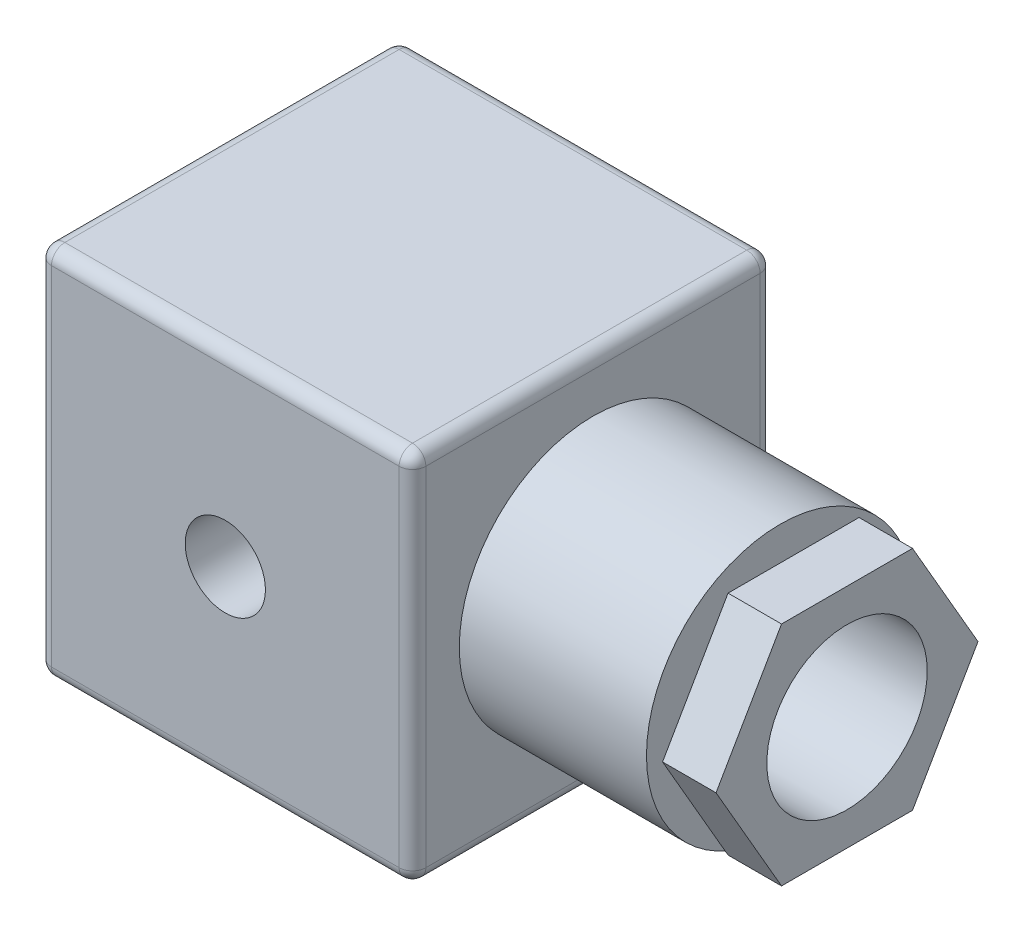
SolidWorks part; units mm, degrees
ref_plane "Front Plane" through (0, 0, 0) normal (0, 0, 1) x (1, 0, 0)
ref_plane "Top Plane" through (0, 0, 0) normal (0, 1, 0) x (1, 0, 0)
ref_plane "Right Plane" through (0, 0, 0) normal (1, 0, 0) x (0, 0, -1)
sketch "Sketch1" plane through (0, 0, 0) normal (0, 0, 1) x (1, 0, 0)
  line L0 (18.5, 7.0716) -> (18.5, 6.292) construction
  line L1 (18.5, 6.292) -> (18.7639, 6.292) construction
  line L2 (18.7639, 6.292) -> (18.7639, 6.6818) construction
  line L3 (18.7639, 6.6818) -> (21.2361, 6.6818) construction
  line L4 (21.2361, 6.6818) -> (21.2361, 6.292) construction
  line L5 (21.2361, 6.292) -> (21.5, 6.292) construction
  line L6 (21.5, 6.292) -> (21.5, 7.0716) construction
  line L7 (21.5, 7.0716) -> (18.5, 7.0716) construction
  line L8 (11.1066, -1.5169) -> (11.1066, 1.5169) construction
  line L9 (11.1066, 1.5169) -> (10.5248, 1.5169) construction
  line L10 (10.5248, 1.5169) -> (10.5248, -1.5169) construction
  line L11 (10.5248, -1.5169) -> (11.1066, -1.5169) construction
  line L12 (18.5, -6.292) -> (18.5, -7.0716) construction
  line L13 (18.5, -7.0716) -> (21.5, -7.0716) construction
  line L14 (21.5, -7.0716) -> (21.5, -6.292) construction
  line L15 (21.5, -6.292) -> (21.2361, -6.292) construction
  line L16 (21.2361, -6.292) -> (21.2361, -6.6818) construction
  line L17 (21.2361, -6.6818) -> (18.7639, -6.6818) construction
  line L18 (18.7639, -6.6818) -> (18.7639, -6.292) construction
  line L19 (18.7639, -6.292) -> (18.5, -6.292) construction
  line L20 (18.5, 7.0716) -> (18.5, 6.292)
  line L21 (18.5, 6.292) -> (18.7639, 6.292)
  line L22 (18.7639, 6.292) -> (18.7639, 6.6818)
  line L23 (18.7639, 6.6818) -> (21.2361, 6.6818)
  line L24 (21.2361, 6.6818) -> (21.2361, 6.292)
  line L25 (21.2361, 6.292) -> (21.5, 6.292)
  line L26 (21.5, 6.292) -> (21.5, 7.0716)
  line L27 (21.5, 7.0716) -> (18.5, 7.0716)
  line L28 (11.1066, -1.5169) -> (11.1066, 1.5169)
  line L29 (11.1066, 1.5169) -> (10.5248, 1.5169)
  line L30 (10.5248, 1.5169) -> (10.5248, -1.5169)
  line L31 (10.5248, -1.5169) -> (11.1066, -1.5169)
  line L32 (18.5, -6.292) -> (18.5, -7.0716)
  line L33 (18.5, -7.0716) -> (21.5, -7.0716)
  line L34 (21.5, -7.0716) -> (21.5, -6.292)
  line L35 (21.5, -6.292) -> (21.2361, -6.292)
  line L36 (21.2361, -6.292) -> (21.2361, -6.6818)
  line L37 (21.2361, -6.6818) -> (18.7639, -6.6818)
  line L38 (18.7639, -6.6818) -> (18.7639, -6.292)
  line L39 (18.7639, -6.292) -> (18.5, -6.292)
  line L40 (17, -6) -> (17, 6) construction
  line L41 (3, 14) -> (31, 14)
  line L42 (3, 14) -> (3, -14)
  line L43 (3, -14) -> (31, -14)
  line L44 (31, 14) -> (31, -14)
  line L45 (3, 14) -> (31, -14) construction
  line L46 (3, -14) -> (31, 14) construction
  point P2 (17, 0)
extrude "Boss-Extrude1" add sketch "Sketch1" along normal blind 27
sketch "Sketch2" plane through (0, 0, 27) normal (0, 0, 1) x (1, 0, 0)
  line L1 (31, 14) -> (3, 14)
  line L2 (31, 14) -> (31, -14)
  line L3 (31, -14) -> (3, -14)
  line L4 (3, 14) -> (3, -14)
extrude "Boss-Extrude2" add sketch "Sketch2" against normal blind 2
sketch "Sketch3" plane through (0, 0, 27) normal (0, 0, 1) x (1, 0, 0)
  circle A0 centre (17, 0) radius 3
extrude "Cut-Extrude1" cut sketch "Sketch3" against normal blind 6
sketch "Sketch4" plane through (0, 0, 21) normal (0, 0, 1) x (1, 0, 0)
  circle A0 centre (17, 0) radius 1.5
extrude "Cut-Extrude2" cut sketch "Sketch4" against normal blind 25
fillet "Fillet1" radius 1 12 edges at (31, 0, 27) (31, 0, 0) (17, -14, 27) (31, -14, 13.5) (17, -14, 0) (31, 14, 13.5) (17, 14, 27) (17, 14, 0) (3, 14, 13.5) (3, 0, 27) (3, -14, 13.5) (3, 0, 0)
sketch "Sketch5" plane through (31, 0, 0) normal (1, 0, 0) x (0, 0, -1)
  circle A0 centre (-13.5, 0) radius 10
extrude "Extrude-Thin1" add sketch "Sketch5" along normal blind 15 thin thin type one direction reverse wall 5
sketch "Sketch6" plane through (46, 0, 0) normal (1, 0, 0) x (0, 0, -1)
  line L1 (-23.2964, 0) -> (-18.3982, -8.484)
  line L2 (-18.3982, -8.484) -> (-8.6018, -8.484)
  line L3 (-8.6018, -8.484) -> (-3.7036, 0)
  line L4 (-3.7036, 0) -> (-8.6018, 8.484)
  line L5 (-8.6018, 8.484) -> (-18.3982, 8.484)
  line L6 (-18.3982, 8.484) -> (-23.2964, 0)
  circle A0 centre (-13.5, 0) radius 8.484 construction
extrude "Boss-Extrude3" add sketch "Sketch6" along normal blind 4
sketch "Sketch7" plane through (46, 0, 0) normal (1, 0, 0) x (0, 0, -1)
  circle A0 centre (-13.5, 0) radius 10
  circle A1 centre (-13.5, 0) radius 7
extrude "Cut-Extrude3" cut sketch "Sketch7" against normal blind 1
sketch "Sketch8" plane through (50, 0, 0) normal (1, 0, 0) x (0, 0, -1)
  circle A0 centre (-13.5, 0) radius 6
extrude "Cut-Extrude4" cut sketch "Sketch8" against normal blind 22
sketch "Sketch9" plane through (0, 0, 0) normal (0, 0, -1) x (-1, 0, 0)
  line L1 (-12.7651, 4.4723) -> (-21.2349, 4.4723)
  line L2 (-12.7651, 4.4723) -> (-12.7651, -4.4723)
  line L3 (-12.7651, -4.4723) -> (-21.2349, -4.4723)
  line L4 (-21.2349, 4.4723) -> (-21.2349, -4.4723)
  line L5 (-12.7651, 4.4723) -> (-21.2349, -4.4723) construction
  line L6 (-12.7651, -4.4723) -> (-21.2349, 4.4723) construction
  point P0 (-17, 0)
extrude "Cut-Extrude5" cut sketch "Sketch9" against normal blind 15
